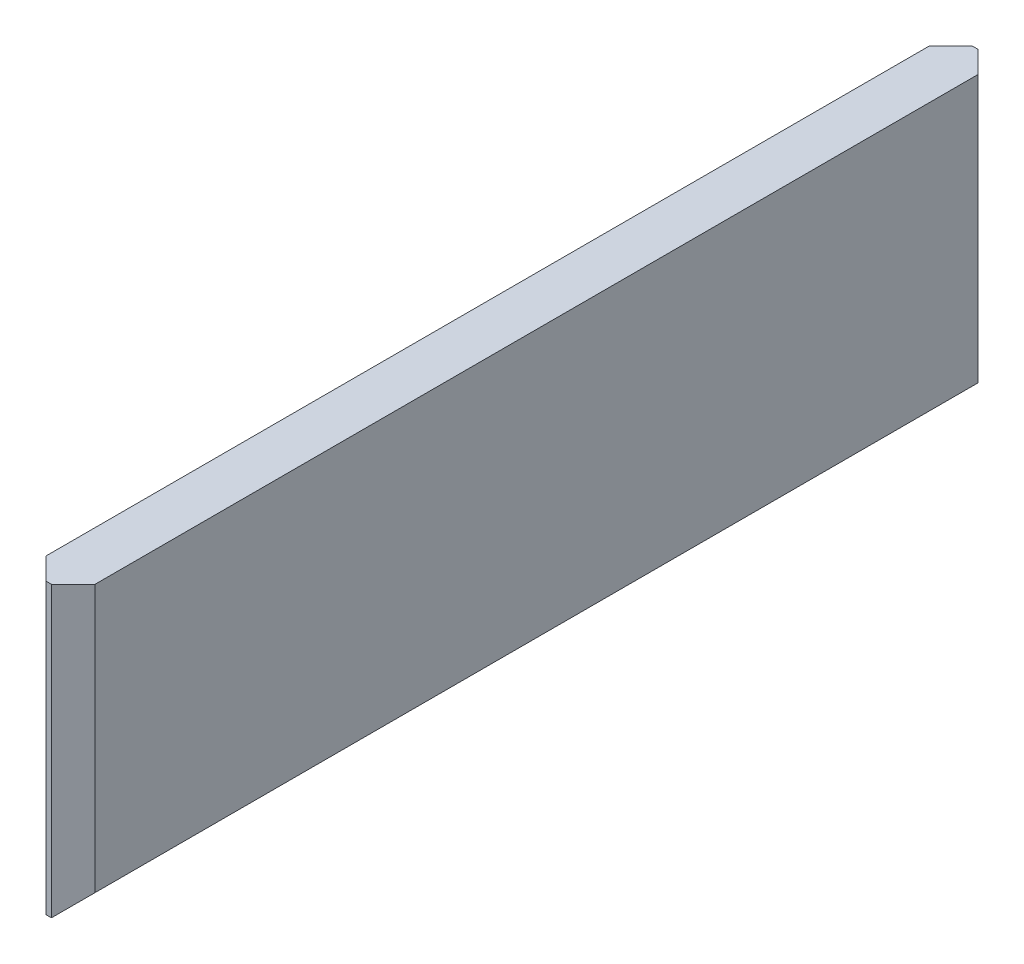
SolidWorks part; units mm, degrees
material "Q235-A"
ref_plane "Front Plane" through (0, 0, 0) normal (0, 0, 1) x (1, 0, 0)
ref_plane "Top Plane" through (0, 0, 0) normal (0, 1, 0) x (1, 0, 0)
ref_plane "Right Plane" through (0, 0, 0) normal (1, 0, 0) x (0, 0, -1)
sketch "Sketch1" plane through (0, 0, 0) normal (1, 0, 0) x (0, 0, -1)
  line L1 (425, -132.5) -> (-425, -132.5)
  line L2 (425, -132.5) -> (425, 132.5)
  line L3 (425, 132.5) -> (-425, 132.5)
  line L4 (-425, -132.5) -> (-425, 132.5)
  line L5 (425, -132.5) -> (-425, 132.5) construction
  line L6 (425, 132.5) -> (-425, -132.5) construction
  point P0 (0, 0)
  dimension "D1" = 850
  dimension "D2" = 265
extrude "Boss-Extrude1" add sketch "Sketch1" along normal mid plane 45
chamfer "Chamfer1" distance 20 angle 45 6 edges at (-22.5, 0, 425) (22.5, 0, 425) (-22.5, 0, -425) (-22.5, -132.5, 0) (22.5, 0, -425) (22.5, -132.5, 0)
